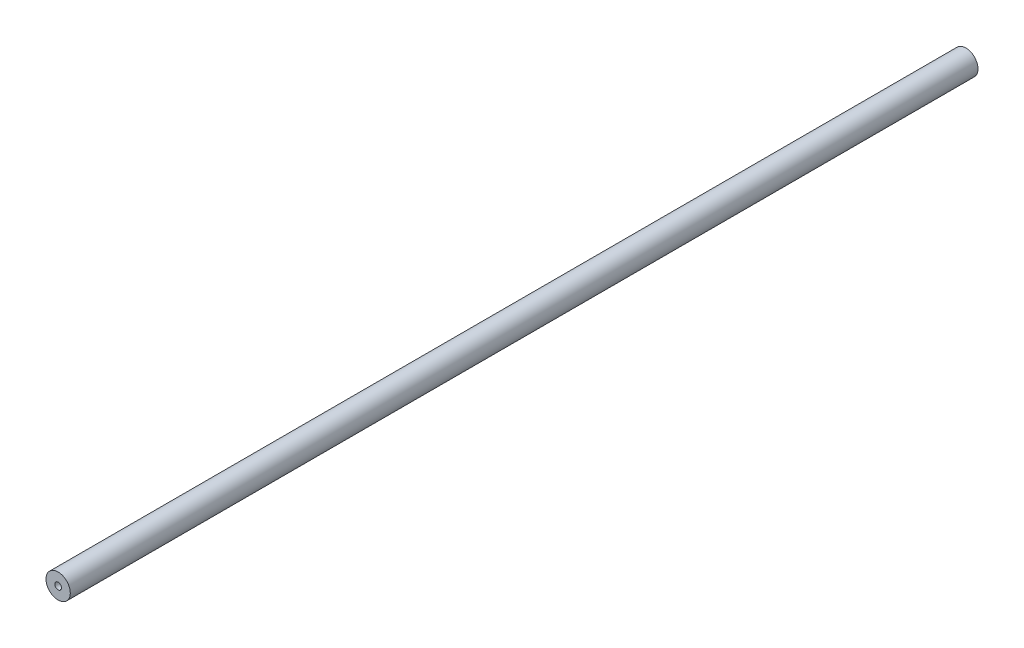
SolidWorks part; units mm, degrees
ref_plane "前视基准面" through (0, 0, 0) normal (0, 0, 1) x (1, 0, 0)
ref_plane "上视基准面" through (0, 0, 0) normal (0, 1, 0) x (1, 0, 0)
ref_plane "右视基准面" through (0, 0, 0) normal (1, 0, 0) x (0, 0, -1)
sketch "草图1" plane through (0, 0, 0) normal (0, 0, 1) x (1, 0, 0)
  circle A0 centre (0, 0) radius 6
  dimension "D1" = 12
extrude "凸台-拉伸1" add sketch "草图1" along normal blind 448
hole_wizard "M4 螺纹孔1" positions "草图3" profile "草图2" tap size "M4" standard "Iso"
sketch "草图3" plane through (0, 0, 0) normal (0, 0, -1) x (-1, 0, 0)
  point P0 (0, 0)
sketch "草图2" plane through (0, 0, 0) normal (1, 0, 0) x (0, 1, 0)
  line L0 (0, 0) -> (0, 15.9914)
  line L1 (0, 15.9914) -> (1.65, 15)
  line L2 (1.65, 15) -> (1.65, 0)
  line L5 (1.65, 0) -> (0, 0)
  line L10 (0, 15.9914) -> (-1.65, 15) construction
  line L11 (0, -6.35) -> (0, 107.95) construction
  dimension "螺纹孔钻头直径" = 3.3
  dimension "螺纹孔钻头深度" = 15
  dimension "导头角度" = 118
cosmetic thread "孔螺蚊线1"
hole_wizard "M4 螺纹孔2" positions "草图5" profile "草图4" tap size "M4" standard "Iso"
sketch "草图5" plane through (0, 0, 448) normal (0, 0, 1) x (1, 0, 0)
  point P0 (0, 0)
sketch "草图4" plane through (0, 0, 448) normal (1, 0, 0) x (0, -1, 0)
  line L0 (0, 0) -> (0, 15.9914)
  line L1 (0, 15.9914) -> (1.65, 15)
  line L2 (1.65, 15) -> (1.65, 0)
  line L5 (1.65, 0) -> (0, 0)
  line L10 (0, 15.9914) -> (-1.65, 15) construction
  line L11 (0, -6.35) -> (0, 107.95) construction
  dimension "螺纹孔钻头直径" = 3.3
  dimension "螺纹孔钻头深度" = 15
  dimension "导头角度" = 118
cosmetic thread "孔螺蚊线2"
